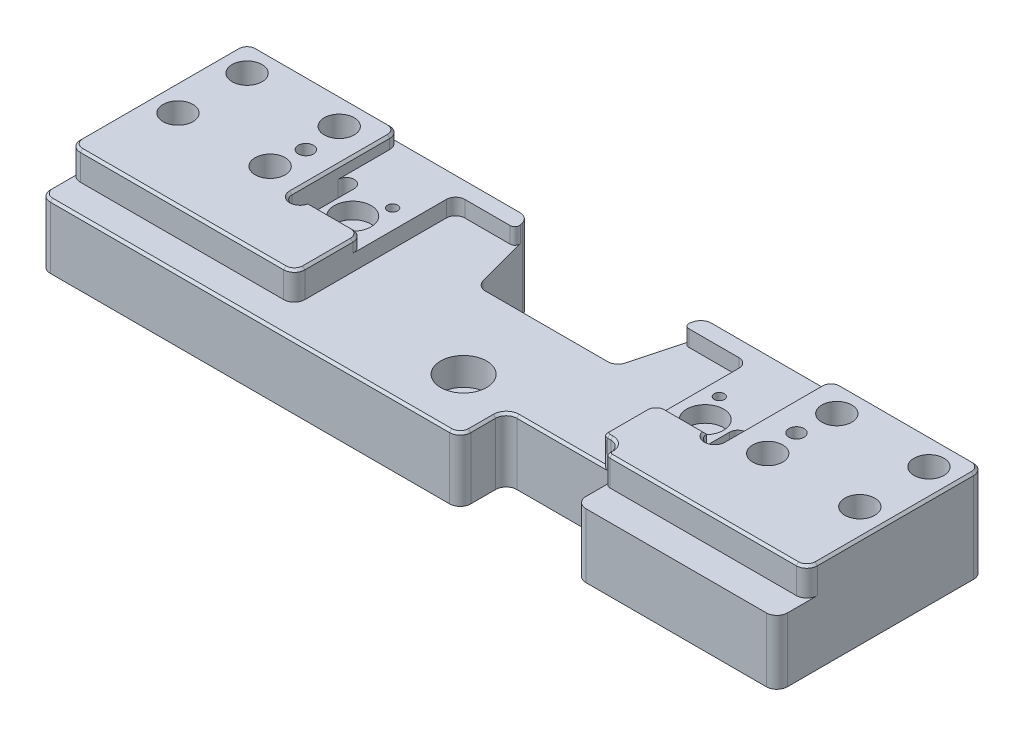
SolidWorks part; units mm, degrees
material "黑电木"
ref_plane "Front Plane" through (0, 0, 0) normal (0, 0, 1) x (1, 0, 0)
ref_plane "Top Plane" through (0, 0, 0) normal (0, 1, 0) x (1, 0, 0)
ref_plane "Right Plane" through (0, 0, 0) normal (1, 0, 0) x (0, 0, -1)
sketch "Sketch1" plane through (0, 0, 0) normal (0, 1, 0) x (1, 0, 0)
  line L1 (-80, -22.5) -> (80, -22.5)
  line L2 (-80, -22.5) -> (-80, 22.5)
  line L3 (-80, 22.5) -> (80, 22.5)
  line L4 (80, -22.5) -> (80, 22.5)
  line L5 (-80, -22.5) -> (80, 22.5) construction
  line L6 (-80, 22.5) -> (80, -22.5) construction
  point P0 (0, 0)
  dimension "D1" = 160
  dimension "D2" = 45
extrude "Boss-Extrude1" add sketch "Sketch1" along normal blind 20
sketch "Sketch2" plane through (0, 20, 0) normal (0, 1, 0) x (1, 0, 0)
  line L0 (80, 22.5) -> (-80, 22.5) construction
  line L1 (-46.75, 22.5) -> (46.75, 22.5)
  line L2 (-46.75, 22.5) -> (-46.75, -1)
  line L3 (-46.75, -1) -> (46.75, -1)
  line L4 (46.75, 22.5) -> (46.75, -1)
  line L5 (0, 22.5) -> (0, 70.127) construction
  dimension "D1" = 93.5
  dimension "D3" = 23.5
extrude "Cut-Extrude1" cut sketch "Sketch2" against normal blind 2.6
sketch "Sketch9" plane through (0, 17.4, 0) normal (0, 1, 0) x (1, 0, 0)
  line L0 (-38.25, 21.5) -> (-38.25, 12.35) construction
  line L5 (-46.75, -1) -> (46.75, -1) construction
  line L14 (-29.25, -1) -> (30.25, -1)
  line L15 (-31.25, 1) -> (-31.25, 17)
  line L16 (-29.25, 19) -> (30.25, 19)
  line L17 (32.25, 1) -> (32.25, 17)
  line L20 (38.25, 12.35) -> (38.25, 21.5) construction
  arc A0 (30.25, -1) -> (32.25, 1) centre (30.25, 1) ccw
  arc A1 (-31.25, 17) -> (-29.25, 19) centre (-29.25, 17) cw
  arc A2 (30.25, 19) -> (32.25, 17) centre (30.25, 17) cw
  arc A3 (-29.25, -1) -> (-31.25, 1) centre (-29.25, 1) cw
  point P17 (-31.25, 19)
  point P22 (-31.25, -1)
  dimension "D4" = 2
  dimension "D1" = 7
  dimension "D2" = 6
  dimension "D3" = 20
extrude "Cut-Extrude14" cut sketch "Sketch9" against normal blind 3.5
sketch "Sketch12" plane through (0, 20, 0) normal (0, 1, 0) x (1, 0, 0)
  line L0 (0, 0) -> (0, 50000) construction
  line L1 (-19.0192, 22.5) -> (-15, 7.5)
  line L3 (-15, 7.5) -> (15, 7.5)
  line L4 (15, 7.5) -> (19.0192, 22.5)
  line L5 (19.0192, 22.5) -> (-19.0192, 22.5)
  line L6 (80, 22.5) -> (46.75, 22.5) construction
  dimension "D1" = 30
  dimension "D2" = 15
  dimension "D3" = 30
extrude "Cut-Extrude7" cut sketch "Sketch12" against normal through all
sketch "Sketch24" plane through (0, 17.4, 0) normal (0, 1, 0) x (1, 0, 0)
  line L0 (-46.75, 22.5) -> (-46.75, -1) construction
  line L1 (-46.75, 9) -> (-43.25, 9)
  line L2 (-46.75, 9) -> (-46.75, -1)
  line L3 (-46.75, -1) -> (-43.25, -1)
  line L4 (-43.25, 9) -> (-43.25, -1)
  line L5 (-46.75, -1) -> (46.75, -1) construction
  line L6 (46.75, -1) -> (46.75, 22.5) construction
  line L7 (46.75, 4) -> (43.25, 4)
  line L8 (46.75, 4) -> (46.75, -1)
  line L9 (46.75, -1) -> (43.25, -1)
  line L10 (43.25, 4) -> (43.25, -1)
  circle A0 centre (-38.25, 3.675) radius 4
  circle A1 centre (38.25, 3.675) radius 4
  dimension "D1" = 8
  dimension "D2" = 5
  dimension "D3" = 3.5
  dimension "D4" = 3.5
  dimension "D5" = 10
extrude "Cut-Extrude16" cut sketch "Sketch24" against normal blind 3.5
sketch "Sketch25" plane through (0, 13.9, 0) normal (0, 1, 0) x (1, 0, 0)
  line L0 (-31.25, 17) -> (-31.25, 1) construction
  line L1 (-31.25, 4) -> (32.25, 4)
  line L2 (-31.25, 4) -> (-31.25, -16)
  line L4 (32.25, 4) -> (32.25, -16)
  line L6 (32.25, 1) -> (32.25, 17) construction
  line L7 (80, -22.5) -> (80, 22.5) construction
  line L9 (-80, -22.5) -> (-80, -16)
  line L10 (-80, -16) -> (-31.25, -16)
  line L11 (80, -22.5) -> (80, -16)
  line L12 (30.25, -1) -> (43.25, -1) construction
  line L13 (-80, -22.5) -> (80, -22.5)
  line L15 (32.25, -16) -> (80, -16)
  line L16 (-29.25, -1) -> (30.25, -1) construction
  dimension "D1" = 15
  dimension "D2" = 5
extrude "Cut-Extrude17" cut sketch "Sketch25" along normal blind 10
sketch "Sketch23" plane through (0, 17.4, 0) normal (0, 1, 0) x (1, 0, 0)
  line L0 (-46.75, -1) -> (-31.25, -1) construction
  line L1 (32.25, -1) -> (46.75, -1) construction
  line L4 (-43.25, -1) -> (-43.25, 9) construction
  line L5 (-46.75, 22.5) -> (-46.75, -1) construction
  line L6 (-43.25, 9) -> (-46.75, 9) construction
  line L7 (46.75, 4) -> (43.25, 4) construction
  circle A0 centre (-45, -1) radius 1.75
  circle A1 centre (45, -1) radius 1.75
  circle A4 centre (-45, 9) radius 1.75
  circle A5 centre (45, 4) radius 1.75
extrude "Cut-Extrude15" cut sketch "Sketch23" along normal blind 10 and the other way up to surface other way up to face at (-45, 13.9, -4)
sketch "Sketch26" plane through (0, 17.4, 0) normal (0, 1, 0) x (1, 0, 0)
  line L0 (-34.25, 8.85) -> (-34.25, 10.85) construction
  line L1 (-36.95, 8.35) -> (-34.6, 8.35) construction
  line L2 (34.25, 10.85) -> (34.25, 8.85) construction
  line L3 (36.95, 8.35) -> (34.6, 8.35) construction
  circle A0 centre (-35.45, 9.55) radius 1.2 construction
  circle A1 centre (35.45, 9.55) radius 1.2 construction
  circle A2 centre (35.45, 9.55) radius 1.1
  circle A3 centre (-35.45, 9.55) radius 1.1
  dimension "D1" = 2.4
  dimension "D2" = 2.4
  dimension "D3" = 2.2
  dimension "D4" = 2.2
extrude "Cut-Extrude18" cut sketch "Sketch26" against normal blind 12
sketch "Sketch29" plane through (0, 20, 0) normal (0, 1, 0) x (1, 0, 0)
  line L0 (0, -22.5) -> (0, 33.7218) construction
  line L1 (-74, 16.5) -> (-54, 16.5) construction
  line L2 (-74, 16.5) -> (-74, 1.5) construction
  line L3 (-74, 1.5) -> (-54, 1.5) construction
  line L4 (-54, 16.5) -> (-54, 1.5) construction
  line L5 (-74, 16.5) -> (-54, 1.5) construction
  line L6 (-74, 1.5) -> (-54, 16.5) construction
  line L7 (-80, -22.5) -> (80, -22.5) construction
  line L8 (-80, 22.5) -> (-80, -16) construction
  line L9 (-46.75, 22.5) -> (-80, 22.5) construction
  line L10 (74, 1.5) -> (54, 16.5) construction
  line L11 (74, 16.5) -> (54, 1.5) construction
  line L12 (54, 16.5) -> (54, 1.5) construction
  line L13 (74, 1.5) -> (54, 1.5) construction
  line L14 (74, 16.5) -> (74, 1.5) construction
  line L15 (74, 16.5) -> (54, 16.5) construction
  point P0 (-64, 9)
  point P18 (64, 9)
  dimension "D1" = 20
  dimension "D2" = 15
  dimension "D3" = 6
  dimension "D4" = 6
hole_wizard "CBORE for M3 Hex Socket Head Cap Screw1" positions "Sketch30" profile "Sketch31" counterbore size "M3" standard "ISO" end condition through all
sketch "Sketch30" plane through (0, 20, 0) normal (0, 1, 0) x (1, 0, 0)
  point P0 (-74, 16.5)
  point P3 (-74, 1.5)
  point P6 (-54, 1.5)
  point P9 (-54, 16.5)
  point P12 (54, 16.5)
  point P15 (54, 1.5)
  point P18 (74, 1.5)
  point P21 (74, 16.5)
sketch "Sketch31" plane through (-74, 20, -16.5) normal (1, 0, 0) x (0, 0, 1)
  line L0 (0, 0) -> (0, 20)
  line L1 (0, 20) -> (1.7, 20)
  line L3 (1.7, 20) -> (1.7, 12.9)
  line L4 (1.7, 12.9) -> (3.25, 12.9)
  line L5 (3.25, 12.9) -> (3.25, 0)
  line L7 (3.25, 0) -> (0, 0)
  line L11 (0, -6.35) -> (0, 107.95) construction
  dimension "通孔孔直径" = 3.4
  dimension "通孔孔深度" = 20
  dimension "柱形沉头孔直径" = 6.5
  dimension "柱形沉头孔深度" = 12.9
sketch "Sketch32" plane through (0, 13.9, 0) normal (0, 1, 0) x (1, 0, 0)
  line L1 (-19.0192, 22.5) -> (-46.75, 22.5) construction
  line L2 (80, -16) -> (80, 22.5) construction
  circle A0 centre (0, -10.5) radius 2.525
  dimension "D1" = 5.05
  dimension "D2" = 33
  dimension "D3" = 80
extrude "Cut-Extrude19" cut sketch "Sketch32" against normal blind 30
hole_wizard "M4 Tapped Hole1" positions "Sketch33" profile "Sketch34" tap size "M4" standard "ISO" end condition through all
sketch "Sketch33" plane through (0, 20, 0) normal (0, 1, 0) x (1, 0, 0)
  line L0 (-43.25, -1) -> (-31.25, -1) construction
  line L3 (-46.75, 22.5) -> (-46.75, -1) construction
  line L4 (46.75, 4) -> (46.75, 22.5) construction
  point P0 (53.25, 8.5)
  point P2 (-53.25, 8.5)
  dimension "D1" = 9.5
  dimension "D2" = 6.5
  dimension "D3" = 6.5
sketch "Sketch34" plane through (53.25, 20, -8.5) normal (1, 0, 0) x (0, 0, 1)
  line L0 (0, 0) -> (0, 20)
  line L1 (0, 20) -> (1.65, 20)
  line L2 (1.65, 20) -> (1.65, 0)
  line L5 (1.65, 0) -> (0, 0)
  line L11 (0, -6.35) -> (0, 107.95) construction
  dimension "通孔螺纹孔钻头直径" = 3.3
  dimension "通孔螺纹孔钻头深度" = 20
cosmetic thread "Cosmetic thread1" parameters "D2"=4
cosmetic thread "Cosmetic thread2" parameters "D2"=4
sketch "Sketch35" plane through (0, 13.9, 0) normal (0, 1, 0) x (1, 0, 0)
  circle A0 centre (0, -10.5) radius 5
  dimension "D1" = 10
extrude "Cut-Extrude20" cut sketch "Sketch35" against normal offset from surface (6 mm away) 7.9 up to face at (53.25, 0, -6.85)
sketch "Sketch36" plane through (0, 13.9, 0) normal (0, 1, 0) x (1, 0, 0)
  line L0 (-80, -22.5) -> (80, -22.5) construction
  line L1 (11.25, -22.5) -> (36.25, -22.5)
  line L2 (11.25, -22.5) -> (11.25, -12.5)
  line L3 (11.25, -12.5) -> (36.25, -12.5)
  line L4 (36.25, -22.5) -> (36.25, -12.5)
  line L6 (32.25, -16) -> (32.25, -1) construction
  dimension "D1" = 25
  dimension "D2" = 10
  dimension "D3" = 4
extrude "Cut-Extrude21" cut sketch "Sketch36" against normal blind 15 and the other way blind 10
fillet "Fillet1" radius 2.3 19 edges at (32.25, 18.7, 1) (46.75, 18.7, -22.5) (-46.75, 18.7, -22.5) (-31.25, 18.7, 1) (-80, 16.95, 16) (80, 16.95, 16) (-31.25, 16.95, 16) (36.25, 6.95, 22.5) (80, 6.95, 22.5) (80, 10, -22.5) (19.0192, 8.7, -22.5) (15, 6.95, -7.5) (-15, 6.95, -7.5) (-19.0192, 8.7, -22.5) (-80, 10, -22.5) (-80, 6.95, 22.5) (11.25, 6.95, 22.5) (11.25, 6.95, 12.5) (36.25, 10, 12.5)
fillet "Fillet2" radius 1 4 edges at (-18.0814, 15.65, -19) (18.0814, 15.65, -19) (32.25, 16.95, 12.5) (36.25, 16.95, 16)
chamfer "Chamfer1" distance 0.5 angle 45 35 edges at (23.4, 13.9, 12.5) (11.9237, 13.9, 13.1737) (-80, 13.9, 16.95) (11.25, 13.9, 17.5) (-79.3263, 13.9, 21.8263) (10.5763, 13.9, 21.8263) (-34.375, 13.9, 22.5) (-45, 20, 2.75) (-46.75, 20, -9.6) (-47.4237, 20, -21.8263) (-38.4, 20, 1) (-63.375, 20, -22.5) (-31.9237, 20, 1.6737) (-79.3263, 20, -21.8263) (-31.25, 20, 8.5) (-80, 20, -3.25) (-31.9237, 20, 15.3263) (-79.3263, 20, 15.3263) (-55.625, 20, 16) (38.9, 20, 1) (45, 20, 2.75) (32.9237, 20, 1.6737) (46.75, 20, -9.6) (32.25, 20, 7.4) (47.4237, 20, -21.8263) (32.5429, 20, 12.2071) (63.375, 20, -22.5) (33.6, 20, 12.5) (79.3263, 20, -21.8263) (35.5763, 20, 13.1737) (80, 20, -3.25) (36.25, 20, 14.9) (79.3263, 20, 15.3263) (36.5429, 20, 15.7071) (57.475, 20, 16)
